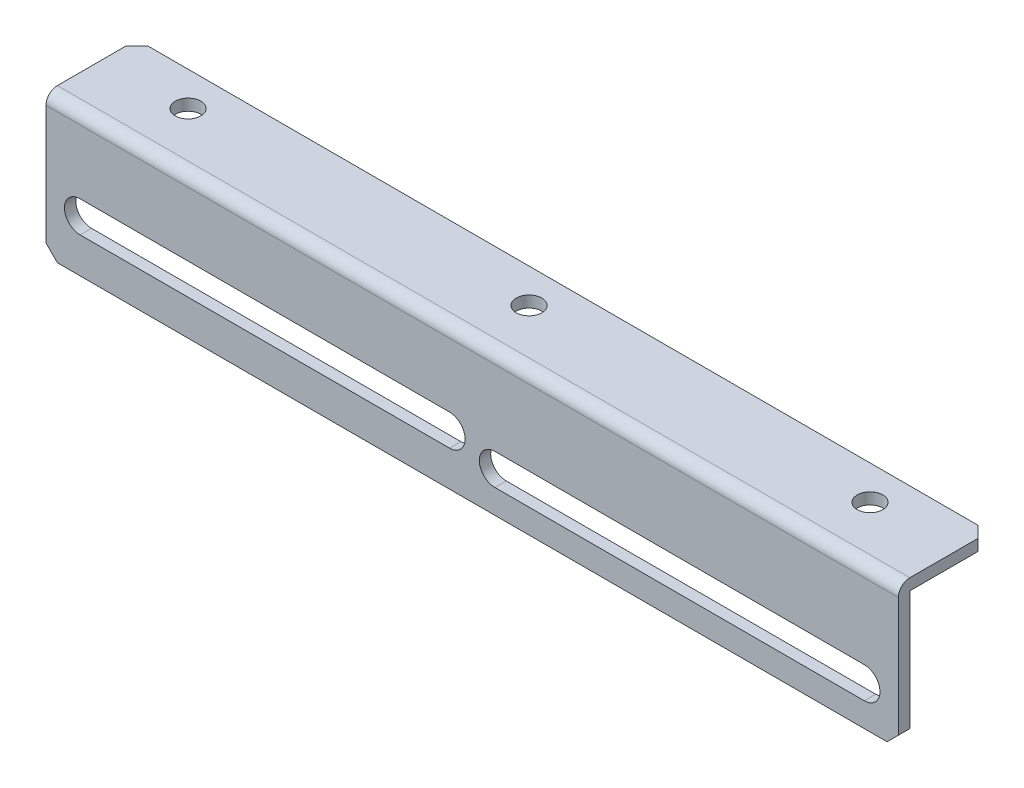
from build123d import *

# Parameters (mm, degrees)
SKETCH_1_W             = 150
SKETCH_1_H             = 25
BOSS_EXTRUDE_1_DEPTH   = 18
SKETCH_2_W             = 16
SKETCH_2_H             = 23
CUT_EXTRUDE_1_DEPTH    = 152.592381075
CUT_EXTRUDE_2_DEPTH    = 78.699742599
CUT_EXTRUDE_3_DEPTH    = 79.136099212
F_4_5_4_5_HOLE_1_D     = 4.5
F_4_5_4_5_HOLE_1_DEPTH = 15
F_4_5_4_5_HOLE_1_TIP   = 1.351936393
F_4_5_4_5_HOLE_3_D     = 4.5
F_4_5_4_5_HOLE_3_DEPTH = 15
F_4_5_4_5_HOLE_3_TIP   = 1.351936393
F_4_5_4_5_HOLE_2_D     = 4.5
F_4_5_4_5_HOLE_2_DEPTH = 15
F_4_5_4_5_HOLE_2_TIP   = 1.351936393
CHAMFER_1_SIZE         = 2
CHAMFER_3_SIZE         = 2
FILLET_1_R             = 2
SKETCH_11_W            = 150
SKETCH_11_H            = 2
CUT_EXTRUDE_4_DEPTH    = 10
CHAMFER_4_SIZE         = 2


with BuildPart() as part:
    # Sketch 1 → Boss-Extrude 1 (new body)
    with BuildSketch(Plane(origin=(0, 0, 0), x_dir=(-1, 0, 0), z_dir=(0, 0, -1))):
        Rectangle(SKETCH_1_W, SKETCH_1_H)
    extrude(amount=-BOSS_EXTRUDE_1_DEPTH)

    # Sketch 2 → Cut-Extrude 1 (cut, through all)
    with BuildSketch(Plane.ZY.offset(75)):
        with Locations((8, -1)):
            Rectangle(SKETCH_2_W, SKETCH_2_H)
    extrude(amount=-CUT_EXTRUDE_1_DEPTH, mode=Mode.SUBTRACT)

    # Sketch 3 → Cut-Extrude 2 (cut, through all)
    with BuildSketch(Plane(origin=(0, 0, 16), x_dir=(-1, 0, 0), z_dir=(0, 0, -1))):
        with BuildLine():
            Line((-4, -2.75), (-69, -2.75))
            ThreePointArc((-69, -2.75), (-71.75, -5.5), (-69, -8.25))
            Line((-69, -8.25), (-4, -8.25))
            ThreePointArc((-4, -8.25), (-1.25, -5.5), (-4, -2.75))
        make_face()
    extrude(amount=-CUT_EXTRUDE_2_DEPTH, mode=Mode.SUBTRACT)

    # Sketch 4 → Cut-Extrude 3 (cut, through all)
    with BuildSketch(Plane.XY.offset(18)):
        with BuildLine():
            Line((-69, -6.25), (-4, -6.25))
            ThreePointArc((-4, -6.25), (-1.25, -3.5), (-4, -0.75))
            Line((-4, -0.75), (-69, -0.75))
            ThreePointArc((-69, -0.75), (-71.75, -3.5), (-69, -6.25))
        make_face()
    extrude(amount=-CUT_EXTRUDE_3_DEPTH, mode=Mode.SUBTRACT)

    # Ø4.5 (4.5) Hole 1
    with Locations(Plane(origin=(0, 12.5, 0), x_dir=(-1, 0, 0), z_dir=(0, 1, 0))):
        with Locations((-60, 8)):
            Hole(F_4_5_4_5_HOLE_1_D / 2, depth=F_4_5_4_5_HOLE_1_DEPTH)
            with Locations((0, 0, -(F_4_5_4_5_HOLE_1_DEPTH + F_4_5_4_5_HOLE_1_TIP / 2))):  # 118° drill point
                Cone(0, F_4_5_4_5_HOLE_1_D / 2, F_4_5_4_5_HOLE_1_TIP, mode=Mode.SUBTRACT)

    # Ø4.5 (4.5) Hole 3
    with Locations(Plane(origin=(0, 12.5, 0), x_dir=(-1, 0, 0), z_dir=(0, 1, 0))):
        with Locations((60, 8)):
            Hole(F_4_5_4_5_HOLE_3_D / 2, depth=F_4_5_4_5_HOLE_3_DEPTH)
            with Locations((0, 0, -(F_4_5_4_5_HOLE_3_DEPTH + F_4_5_4_5_HOLE_3_TIP / 2))):  # 118° drill point
                Cone(0, F_4_5_4_5_HOLE_3_D / 2, F_4_5_4_5_HOLE_3_TIP, mode=Mode.SUBTRACT)

    # Ø4.5 (4.5) Hole 2
    with Locations(Plane(origin=(0, 12.5, 0), x_dir=(-1, 0, 0), z_dir=(0, 1, 0))):
        with Locations((0, 8)):
            Hole(F_4_5_4_5_HOLE_2_D / 2, depth=F_4_5_4_5_HOLE_2_DEPTH)
            with Locations((0, 0, -(F_4_5_4_5_HOLE_2_DEPTH + F_4_5_4_5_HOLE_2_TIP / 2))):  # 118° drill point
                Cone(0, F_4_5_4_5_HOLE_2_D / 2, F_4_5_4_5_HOLE_2_TIP, mode=Mode.SUBTRACT)

    # Chamfer 1
    chamfer_1_edges = [part.edges().sort_by_distance(p)[0] for p in [
        (75, -12.5, 17),
    ]]
    chamfer(chamfer_1_edges, length=CHAMFER_1_SIZE)

    # Chamfer 3
    chamfer_3_edges = [part.edges().sort_by_distance(p)[0] for p in [
        (-75, -12.5, 17),
    ]]
    chamfer(chamfer_3_edges, length=CHAMFER_3_SIZE)

    # Fillet 1
    fillet_1_edges = [part.edges().sort_by_distance(p)[0] for p in [
        (0, 12.5, 18),
    ]]
    fillet(fillet_1_edges, radius=FILLET_1_R)

    # Sketch 11 → Cut-Extrude 4 (cut)
    with BuildSketch(Plane(origin=(0, 12.5, 0), x_dir=(1, 0, 0), z_dir=(0, 1, 0))):
        with Locations((0, -1)):
            Rectangle(SKETCH_11_W, SKETCH_11_H)
    extrude(amount=-CUT_EXTRUDE_4_DEPTH, mode=Mode.SUBTRACT)

    # Chamfer 4
    chamfer_4_edges = [part.edges().sort_by_distance(p)[0] for p in [
        (75, 11.5, 2),
        (-75, 11.5, 2),
    ]]
    chamfer(chamfer_4_edges, length=CHAMFER_4_SIZE)


solid = part.part
